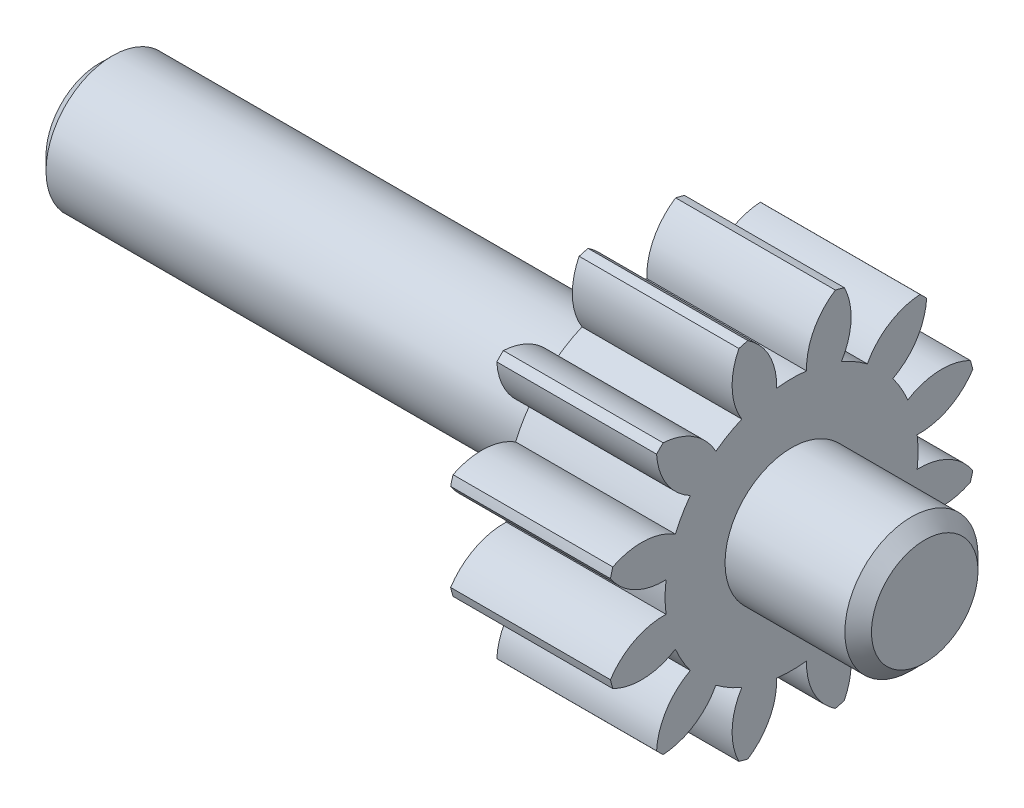
SolidWorks part; units mm, degrees
ref_plane "Plane1" through (0, 0, 0) normal (0, 0, 1) x (1, 0, 0)
ref_plane "Plane2" through (0, 0, 0) normal (0, 1, 0) x (1, 0, 0)
ref_plane "Plane3" through (0, 0, 0) normal (1, 0, 0) x (0, 0, -1)
sketch "HoldingSke" plane through (0, 0, 0) normal (0, 1, 0) x (1, 0, 0)
  line L0 (0, 0) -> (0.9781, -0.2079)
  line L1 (-15, 0) -> (100, 0) construction
  line L2 (0, 0) -> (-2.1039, 2.3779)
  line L3 (0, 0) -> (-11.863, 4.5341)
  line L4 (0, 0) -> (8.4473, 1.7955)
  line L5 (0, 0) -> (-46.8476, -17.4728)
  line L6 (0, 0) -> (-4.9738, -3.3558)
  line L7 (-2.1039, 2.3779) -> (8.6586, 51.2059)
  line L8 (-76.2, 54.61) -> (-76.1, 54.61)
  line L9 (-71.009, 38.7566) -> (-53.1078, 45.2721)
  line L10 (-76.2, 71.12) -> (104.1128, 71.12)
  line L11 (0, 0) -> (-6, 0)
  line L12 (-76.2, 101.6) -> (-76.162, 101.6)
  line L13 (24.9733, 27.94) -> (52.9518, 28.4284)
  line L14 (24.9733, 27.94) -> (24.9743, 27.94)
  line L15 (24.9733, 27.94) -> (100.4006, 29.5858)
  line L16 (-63.627, -1) -> (-12.827, -1)
  circle A0 centre (0, 0) radius 0.4
  circle A1 centre (0, 0) radius 4.749
  circle A2 centre (0, 0) radius 37.5
  circle A3 centre (0, 0) radius 0.4
sketch "BasProSke" plane through (0, 0, 0) normal (0, 1, 0) x (1, 0, 0)
  line L0 (-10, 0) -> (60, 0) construction
  line L1 (0, 0) -> (0, 7)
  line L2 (0, 0) -> (6, 0)
  line L3 (6, 0) -> (6, 7)
  line L4 (6, 7) -> (0, 7)
revolve "Base-Revolve" add sketch "BasProSke" angle 360 about L0
sketch "TooCutSke" plane through (0, 0, 0) normal (1, 0, 0) x (0, 0, -1)
  line L1 (0, 0) -> (0, 107) construction
  line L2 (0, 0) -> (-0.8496, 5.9395) construction
  line L3 (0, 0) -> (-3.0836, 11.5081) construction
  line L4 (-0.8496, 5.9395) -> (-1.5418, 5.7541) construction
  arc A0 (0.5622, 4.7156) -> (-0.5622, 4.7156) centre (0, 0) ccw
  arc A1 (1.6729, 6.8233) -> (-1.6729, 6.8233) centre (0, 0) ccw
  circle A2 centre (0, 0) radius 6 construction
  circle A3 centre (0, 0) radius 5.6382 construction
  arc A4 (-0.5622, 4.7156) -> (-1.6729, 6.8233) centre (-2.9608, 4.7982) ccw
  arc A5 (1.6729, 6.8233) -> (0.5622, 4.7156) centre (2.9608, 4.7982) ccw
extrude "ToothCut" cut sketch "TooCutSke" along normal through all
fillet "Breaks" [suppressed] radius 0.02
fillet "RootFillets" [suppressed] radius 0.251
pattern_circular "TeethCuts" count 12 every 30 about axis through (-10, 0, 0) along (1, 0, 0) of "ToothCut", "RootFillets", "Breaks"
sketch "HubNeaOneSke" plane through (0, 0, 0) normal (-1, 0, 0) x (0, 0, 1)
  circle A0 centre (0, 0) radius 4.749
extrude "HubNearOne" [suppressed] add sketch "HubNeaOneSke" along normal blind 44.0001
sketch "HubNeaBotSke" plane through (0, 0, 0) normal (-1, 0, 0) x (0, 0, 1)
  circle A0 centre (0, 0) radius 4.749
extrude "HubNearBoth" [suppressed] add sketch "HubNeaBotSke" along normal blind 22
ref_plane "FarPln" through (6, 0, 0) normal (1, 0, 0) x (0, 0, -1)
sketch "HubFarSke" plane through (6, 0, 0) normal (1, 0, 0) x (0, 0, -1)
  circle A0 centre (0, 0) radius 4.749
extrude "HubFar" [suppressed] add sketch "HubFarSke" along normal blind 22
sketch "BorSke" plane through (0, 0, 0) normal (1, 0, 0) x (0, 0, -1)
  circle A0 centre (0, 0) radius 0.4
extrude "Bore" cut sketch "BorSke" along normal mid plane 100.0001
sketch "KeySke" plane through (0, 0, 0) normal (1, 0, 0) x (0, 0, -1)
  line L0 (-0.05, 0) -> (-0.05, 0.5)
  line L1 (-0.05, 0.5) -> (0.05, 0.5)
  line L2 (0.05, 0.5) -> (0.05, 0)
  line L3 (0, 0) -> (0, 34) construction
  line L4 (-0.05, 0) -> (0.05, 0)
extrude "Keyway" [suppressed] cut sketch "KeySke" along normal mid plane 100.0001
pattern_circular "Keyway2" [suppressed] count 2 every 90 about axis through (-10, 0, 0) along (1, 0, 0)
sketch "Sketch1" plane through (6, 0, 0) normal (1, 0, 0) x (0, 0, -1)
  circle A0 centre (0, 0) radius 2.5
  dimension "D1" = 5
extrude "Boss-Extrude1" add sketch "Sketch1" along normal blind 5
sketch "Sketch2" plane through (0, 0, 0) normal (-1, 0, 0) x (0, 0, 1)
  circle A0 centre (0, 0) radius 2.5
  dimension "D1" = 5
extrude "Boss-Extrude2" add sketch "Sketch2" along normal blind 20
chamfer "Chamfer1" distance 0.5 angle 45 2 edges at (11, 0, -2.5) (-20, 0, 2.5)
equation "' \"Module@HoldingSke\" = 6.35"
equation "' \"Num_teeth@HoldingSke\" = 12"
equation "' \"Ap@HoldingSke\" =  20"
equation "' \"Ap@HoldingSke\" = 20"
equation "' \"Width@HoldingSke\" = 0.5 * 25.4"
equation "' \"Hub_dia@HoldingSke\"= 1 * 25.4"
equation "' \"Hub_dia@HoldingSke\" = 1 * 25.4"
equation "' \"Overall_len@HoldingSke\" = 1.0 * 25.4"
equation "' \"Bore@HoldingSke\" = 0.75 * 25.4"
equation "' \"T_dim@HoldingSke\" = 0.1 * 25.4"
equation "' \"Width@KeySke\" = 0.25 * 25.4"
equation "' \"Show_teeth@HoldingSke\" = 13"
equation "' \"Backlash@HoldingSke\" = 0.009 * 25.4"
equation "' \"Addendum_fac@HoldingSke\" = 1.0"
equation "' \"Dedendum_fac@HoldingSke\" = 1.25"
equation "' \"Dedendum_add@HoldingSke\" = 0.00005 * 25.4"
equation "' \"Clearance_fac@HoldingSke\" = 0.25"
equation "\"Pitch@HoldingSke\" = 1 / \"Module@HoldingSke\""
equation "\"Overcut_dia@TooCutSke\" = (\"Num_teeth@HoldingSke\" + 2 * \"Addendum_fac@HoldingSke\") / \"Pitch@HoldingSke\" + 0.002 * 25.4"
equation "\"Pitch_dia@TooCutSke\" = \"Num_teeth@HoldingSke\" / \"Pitch@HoldingSke\""
equation "\"Base_dia@TooCutSke\" = \"Num_teeth@HoldingSke\" / \"Pitch@HoldingSke\" * cos((\"Ap@HoldingSke\"  * 3.14159265 / 180))"
equation "\"Root_dia@TooCutSke\" = (\"Num_teeth@HoldingSke\" + 2) / \"Pitch@HoldingSke\" - 2 * (\"Addendum_fac@HoldingSke\" + \"Dedendum_fac@HoldingSke\") / \"Pitch@HoldingSke\" - \"Dedendum_add@HoldingSke\" * 2"
equation "\"Half_ang@TooCutSke\" = 180 / \"Num_teeth@HoldingSke\""
equation "\"Half_CT@TooCutSke\" = \"Num_teeth@HoldingSke\" / \"Pitch@HoldingSke\" * sin((3.14159265 / 2 / \"Num_teeth@HoldingSke\")) / 2 - 7 * \"Backlash@HoldingSke\" / 4"
equation "\"Flank_rad@TooCutSke\" = \"Num_teeth@HoldingSke\" / \"Pitch@HoldingSke\" / 5"
equation "\"Radius@RootFillets\" = \"Clearance_fac@HoldingSke\" / \"Pitch@HoldingSke\" + \"Dedendum_add@HoldingSke\""
equation "\"Break_rad@Breaks\" = 0.02 / \"Pitch@HoldingSke\""
equation "\"Thickness@HoldingSke\" = \"Width@HoldingSke\""
equation "\"OAL@HoldingSke\" = \"Thickness@HoldingSke\""
equation "\"MHD@HoldingSke\" = (\"Num_teeth@HoldingSke\" + 2) / \"Pitch@HoldingSke\" - 2 * (\"Addendum_fac@HoldingSke\" + \"Dedendum_fac@HoldingSke\")  / \"Pitch@HoldingSke\" - \"Dedendum_add@HoldingSke\" * 2"
equation "\"MBD@HoldingSke\" = (\"Num_teeth@HoldingSke\" + 2) / \"Pitch@HoldingSke\" - 2 * (\"Addendum_fac@HoldingSke\" + \"Dedendum_fac@HoldingSke\")  / \"Pitch@HoldingSke\" - \"Dedendum_add@HoldingSke\" * 2 - 0.002 * 25.4"
equation "\"MHD@HoldingSke\" = ((sgn( \"MHD@HoldingSke\" - \"Hub_dia@HoldingSke\" )-1)*( \"MHD@HoldingSke\" - \"Hub_dia@HoldingSke\" ))/-2+ \"Hub_dia@HoldingSke\""
equation "\"MBD@HoldingSke\" = ((sgn( \"MBD@HoldingSke\" - \"Bore@HoldingSke\" )-1)*( \"MBD@HoldingSke\" - \"Bore@HoldingSke\" ))/-2+ \"Bore@HoldingSke\""
equation "\"OAL@HoldingSke\" = ((sgn( \"OAL@HoldingSke\" - \"Overall_len@HoldingSke\" )+1)*( \"OAL@HoldingSke\" - \"Overall_len@HoldingSke\" ))/2 + \"Overall_len@HoldingSke\" + 0.000002 * 25.4"
equation "\"Num_teeth@TeethCuts\" = int( \"Show_teeth@HoldingSke\" ) + 1"
equation "\"Num_teeth@TeethCuts\" = ((sgn( \"Num_teeth@TeethCuts\" - \"Num_teeth@HoldingSke\" )-1)*( \"Num_teeth@TeethCuts\" - \"Num_teeth@HoldingSke\" ))/-2+ \"Num_teeth@HoldingSke\""
equation "\"Num_teeth@TeethCuts\" = ((sgn( \"Num_teeth@TeethCuts\" - 2.0)+1)*( \"Num_teeth@TeethCuts\" - 2.0))/2 +2.0"
equation "\"Angle@TeethCuts\" = 360.0 / \"Num_teeth@HoldingSke\""
equation "\"Diameter@BasProSke\" = (\"Num_teeth@HoldingSke\" + 2 * \"Addendum_fac@HoldingSke\") / \"Pitch@HoldingSke\""
equation "\"Thickness@BasProSke\"  = \"Thickness@HoldingSke\""
equation "' \"Fillet_rad@BasProSke\" =  \"Thickness@HoldingSke\" * 0.05"
equation "' \"Fillet_rad@BasProSke\" = \"Thickness@HoldingSke\" * 0.05"
equation "\"MHD@HoldingSke\" = ((sgn( \"MHD@HoldingSke\" - \"Root_dia@TooCutSke\" )-1)*( \"MHD@HoldingSke\" - \"Root_dia@TooCutSke\" ))/-2+ \"Root_dia@TooCutSke\""
equation "\"Diameter@HubNeaOneSke\" = \"MHD@HoldingSke\""
equation "\"Length@HubNearOne\" = \"OAL@HoldingSke\" - \"Thickness@BasProSke\""
equation "\"Diameter@HubNeaBotSke\" = \"MHD@HoldingSke\""
equation "\"Length@HubNearBoth\" = ( \"OAL@HoldingSke\" - \"Thickness@BasProSke\" ) / 2.0"
equation "\"Thickness@FarPln\" = \"Thickness@BasProSke\""
equation "\"Diameter@HubFarSke\" = \"MHD@HoldingSke\""
equation "\"Length@HubFar\" = ( \"OAL@HoldingSke\" - \"Thickness@BasProSke\" ) / 2.0"
equation "\"Diameter@BorSke\" = \"MBD@HoldingSke\""
equation "\"D1@Bore\" = \"OAL@HoldingSke\" * 2.0"
equation "\"D1@Keyway\" = \"OAL@HoldingSke\" * 2.0"
equation "\"Offset@KeySke\" = \"T_dim@HoldingSke\" + \"MBD@HoldingSke\" / 2.0"
